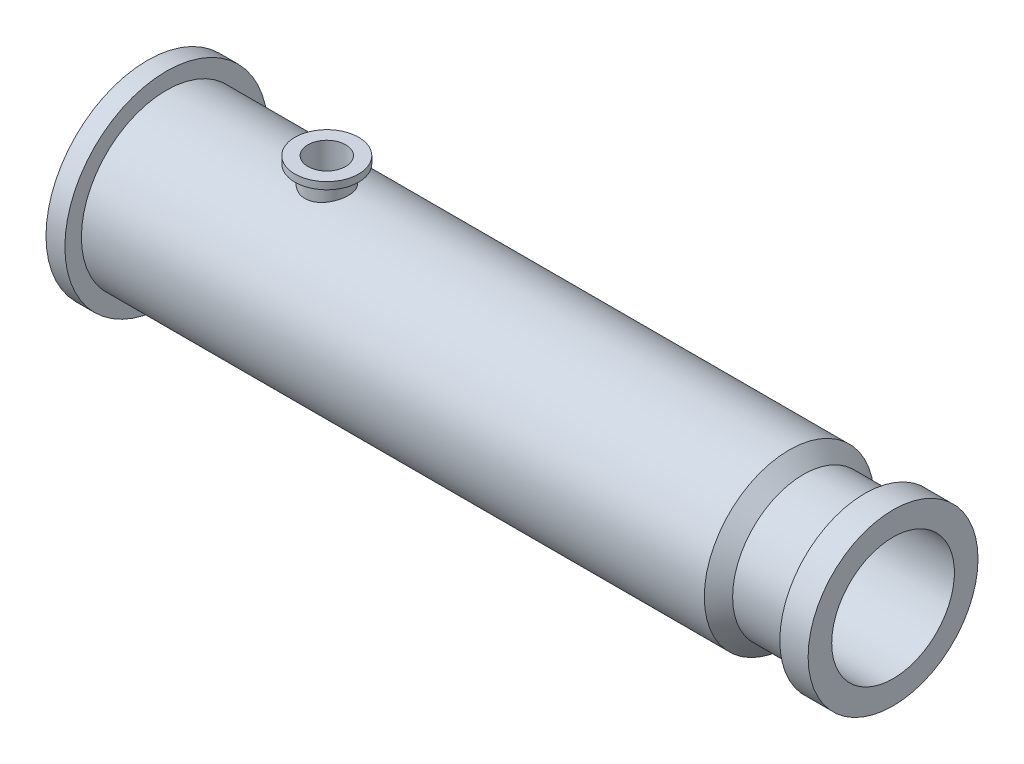
SolidWorks part; units mm, degrees
material "普通碳钢"
ref_plane "Front Plane" through (0, 0, 0) normal (0, 0, 1) x (1, 0, 0)
ref_plane "Top Plane" through (0, 0, 0) normal (0, 1, 0) x (1, 0, 0)
ref_plane "Right Plane" through (0, 0, 0) normal (1, 0, 0) x (0, 0, -1)
sketch "Sketch1" plane through (0, 0, 0) normal (0, 0, 1) x (1, 0, 0)
  line L0 (0, 160) -> (0, 215)
  line L1 (0, 215) -> (40, 215)
  line L2 (40, 215) -> (40, 180)
  line L3 (40, 180) -> (1360, 180)
  line L4 (1360, 180) -> (1390, 150)
  line L5 (1390, 150) -> (1520, 150)
  line L6 (1520, 150) -> (1520, 180)
  line L7 (1520, 180) -> (1580, 180)
  line L8 (1580, 180) -> (1580, 130)
  line L10 (0, 0) -> (1704.8064, 0) construction
  line L11 (1351.7157, 160) -> (1381.7157, 130)
  line L12 (1381.7157, 130) -> (1580, 130)
  line L13 (1351.7157, 160) -> (0, 160)
  dimension "D1" = 1580
  dimension "D2" = 60
  dimension "D3" = 40
  dimension "D4" = 215
  dimension "D5" = 20
  dimension "D6" = 180
  dimension "D7" = 180
  dimension "D8" = 20
  dimension "D9" = 20
  dimension "D10" = 160
  dimension "D11" = 130
  dimension "D12" = 45
revolve "Revolve1" add sketch "Sketch1" angle 360 about L10
sketch "Sketch2" plane through (1580, 0, 0) normal (1, 0, 0) x (0, 0, -1)
  line L0 (0, 0) -> (180, 0) construction
  line L1 (0, 0) -> (0, 180) construction
  circle A0 centre (0, 0) radius 180 construction
sketch "Sketch3" plane through (0, 0, 0) normal (0, 1, 0) x (1, 0, 0)
  line L0 (0, 215) -> (0, -215) construction
  circle A0 centre (380, 0) radius 40
  circle A1 centre (380, 0) radius 46
  dimension "D1" = 80
  dimension "D2" = 92
  dimension "D3" = 380
extrude "Boss-Extrude1" add sketch "Sketch3" along normal blind 215
sketch "Sketch4" plane through (0, 0, 0) normal (-1, 0, 0) x (0, 0, 1)
  circle A0 centre (0, 0) radius 160
extrude "Cut-Extrude1" cut sketch "Sketch4" against normal blind 900
sketch "Sketch5" plane through (0, 215, 0) normal (0, 1, 0) x (1, 0, 0)
  circle A0 centre (380, 0) radius 40
  dimension "D1" = 80
extrude "Cut-Extrude2" cut sketch "Sketch5" against normal blind 300
sketch "Sketch6" plane through (0, 215, 0) normal (0, 1, 0) x (1, 0, 0)
  circle A0 centre (380, 0) radius 40
  circle A1 centre (380, 0) radius 67.5
  dimension "D1" = 135
extrude "Boss-Extrude2" add sketch "Sketch6" along normal blind 15
